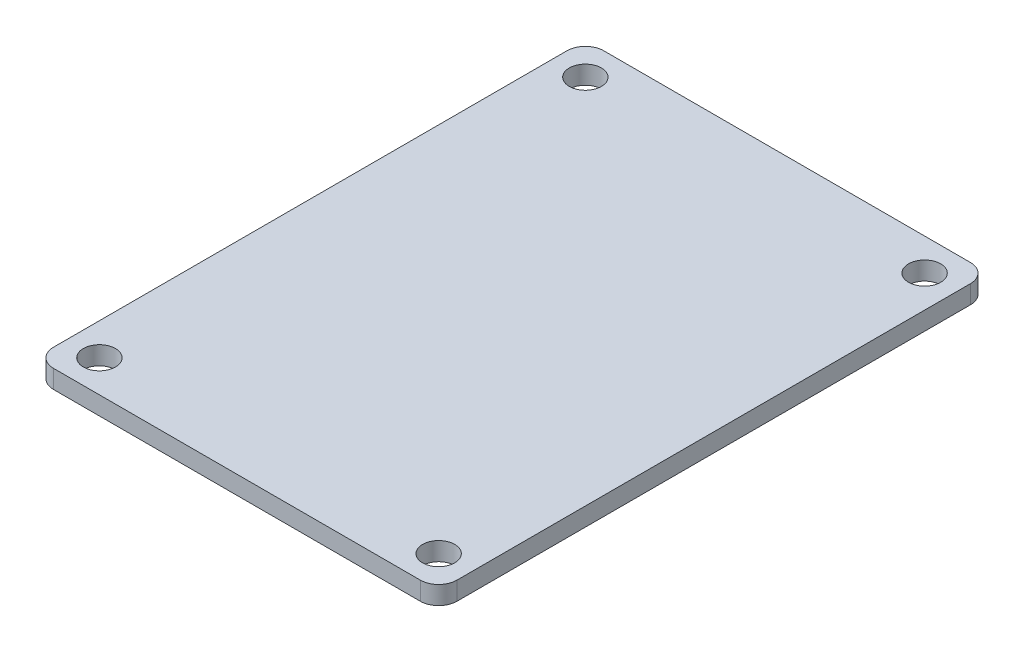
SolidWorks part; units mm, degrees
material "Q235A"
ref_plane "Front Plane" through (0, 0, 0) normal (0, 0, 1) x (1, 0, 0)
ref_plane "Top Plane" through (0, 0, 0) normal (0, 1, 0) x (1, 0, 0)
ref_plane "Right Plane" through (0, 0, 0) normal (1, 0, 0) x (0, 0, -1)
sketch "Sketch1" plane through (0, 0, 0) normal (0, 1, 0) x (1, 0, 0)
  line L1 (-69.85, 95.25) -> (69.85, 95.25)
  line L2 (-69.85, 95.25) -> (-69.85, -95.25)
  line L3 (-69.85, -95.25) -> (69.85, -95.25)
  line L4 (69.85, 95.25) -> (69.85, -95.25)
  dimension "D1" = 95.25
  dimension "D2" = 190.5
  dimension "D3" = 69.85
  dimension "D4" = 139.7
extrude "Boss-Extrude1" add sketch "Sketch1" along normal blind 6.35
fillet "Fillet1" radius 6.35 4 edges at (-69.85, 3.175, -95.25) (69.85, 3.175, -95.25) (69.85, 3.175, 95.25) (-69.85, 3.175, 95.25)
hole_wizard "7/16 (0.4375) Diameter Hole1" positions "Sketch3" profile "Sketch2" hole size "7/16" standard "Ansi Inch" end condition through all
sketch "Sketch3" plane through (0, 6.35, 0) normal (0, 1, 0) x (1, 0, 0)
  line L0 (63.5, 95.25) -> (-63.5, 95.25) construction
  line L2 (-69.85, 88.9) -> (-69.85, -88.9) construction
  point P0 (-58.738, 84.138)
  dimension "D1" = 11.112
  dimension "D2" = 11.112
sketch "Sketch2" plane through (-58.738, 6.35, -84.138) normal (1, 0, 0) x (0, 0, 1)
  line L0 (0, 0) -> (0, 6.35)
  line L1 (0, 6.35) -> (5.5562, 6.35)
  line L2 (5.5562, 6.35) -> (5.5562, 0)
  line L5 (5.5562, 0) -> (0, 0)
  line L11 (0, -6.35) -> (0, 107.95) construction
  dimension "通孔孔直径" = 11.1125
  dimension "通孔孔深度" = 6.35
pattern_linear "LPattern1" count 2 spacing 168.275 along (0, 0, 1) count 2 spacing 117.475 along (1, 0, 0) of "7/16 (0.4375) Diameter Hole1"
